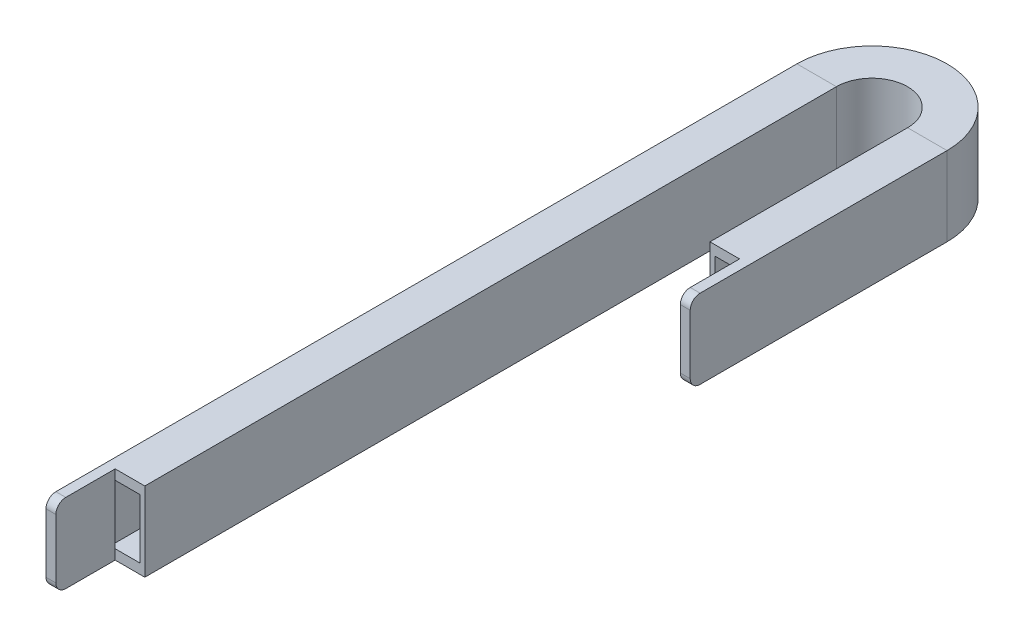
SolidWorks part; units mm, degrees
material "6061"
ref_plane "前视基准面" through (0, 0, 0) normal (0, 0, 1) x (1, 0, 0)
ref_plane "上视基准面" through (0, 0, 0) normal (0, 1, 0) x (1, 0, 0)
ref_plane "右视基准面" through (0, 0, 0) normal (1, 0, 0) x (0, 0, -1)
sketch "草图1" plane through (0, 0, 0) normal (0, 0, 1) x (1, 0, 0)
  line L1 (-10, 20) -> (10, 20)
  line L2 (-10, 20) -> (-10, -20)
  line L3 (-10, -20) -> (10, -20)
  line L4 (10, 20) -> (10, -20)
  line L5 (-10, 20) -> (10, -20) construction
  line L6 (-10, -20) -> (10, 20) construction
  point P0 (0, 0)
  dimension "D1" = 20
  dimension "D2" = 40
sketch "草图2" plane through (0, 0, 0) normal (0, 1, 0) x (1, 0, 0)
  line L0 (0, 0) -> (0, 350)
  line L1 (0, 350) -> (379.3582, 350) construction
  line L2 (56, 350) -> (56, 250)
  arc A0 (56, 350) -> (0, 350) centre (28, 350) ccw
  dimension "D2" = 56
  dimension "D1" = 350
  dimension "D3" = 100
sweep "扫描1" add profiles "草图1" path "草图2"
sketch "草图11" plane through (0, 0, 0) normal (0, 0, 1) x (1, 0, 0)
  line L1 (7.5, 15) -> (-7.5, 15)
  line L2 (7.5, 15) -> (7.5, -15)
  line L3 (7.5, -15) -> (-7.5, -15)
  line L4 (-7.5, 15) -> (-7.5, -15)
  line L5 (7.5, 15) -> (-7.5, -15) construction
  line L6 (7.5, -15) -> (-7.5, 15) construction
  point P0 (0, 0)
  dimension "D1" = 30
  dimension "D2" = 15
sketch "草图12" plane through (0, 0, 0) normal (0, 1, 0) x (1, 0, 0)
  line L0 (0, 0) -> (0, 350)
  line L1 (56, 243.9814) -> (56, 350)
  arc A0 (56, 350) -> (0, 350) centre (28, 350) ccw
  dimension "D1" = 56
sweep "切除-扫描1" cut profiles "草图11" path "草图12"
sketch "草图3" plane through (0, 0, 0) normal (0, 0, 1) x (1, 0, 0)
  line L0 (10, 20) -> (-10, 20) construction
  line L1 (-5, 20) -> (-10, 20)
  line L2 (-5, 20) -> (-5, -20)
  line L3 (-5, -20) -> (-10, -20)
  line L4 (-10, 20) -> (-10, -20)
  dimension "D1" = 5
extrude "凸台-拉伸1" add sketch "草图3" along normal blind 30
fillet "圆角1" radius 5 2 edges at (-7.5, -20, 30) (-7.5, 20, 30)
sketch "草图5" plane through (0, 0, -250) normal (0, 0, 1) x (1, 0, 0)
  line L0 (46, 20) -> (66, 20) construction
  line L1 (66, -20) -> (61, -20)
  line L2 (66, -20) -> (66, 20)
  line L3 (66, 20) -> (61, 20)
  line L4 (61, -20) -> (61, 20)
  dimension "D1" = 5
extrude "凸台-拉伸2" add sketch "草图5" along normal blind 30
fillet "圆角2" radius 5 2 edges at (63.5, 20, -220) (63.5, -20, -220)
